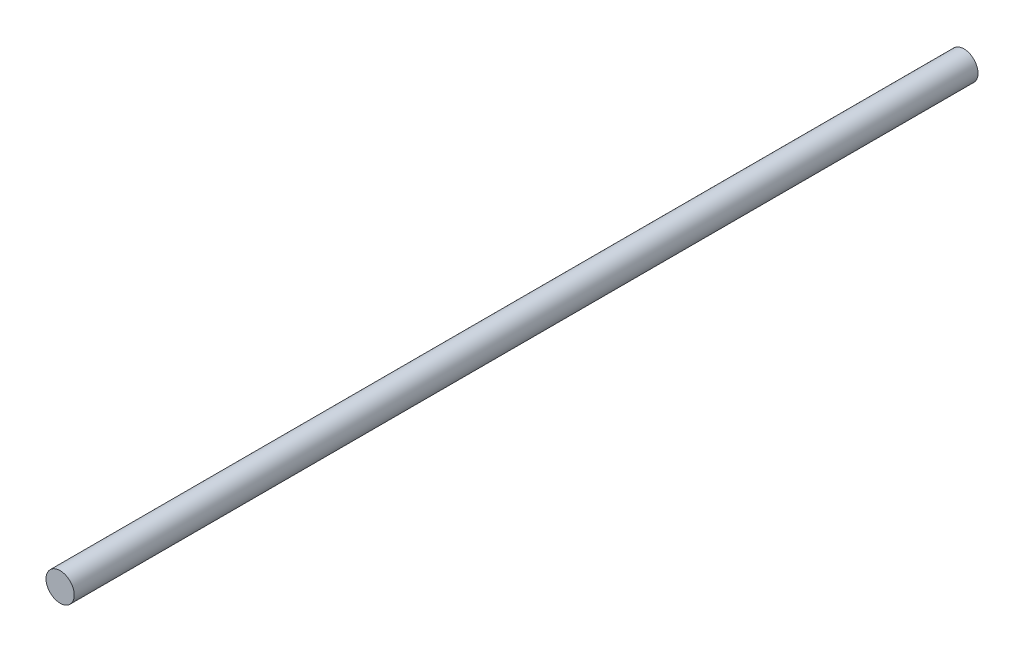
SolidWorks part; units mm, degrees
ref_plane "Front Plane" through (0, 0, 0) normal (0, 0, 1) x (1, 0, 0)
ref_plane "Top Plane" through (0, 0, 0) normal (0, 1, 0) x (1, 0, 0)
ref_plane "Right Plane" through (0, 0, 0) normal (1, 0, 0) x (0, 0, -1)
other "Configuration Table"
sketch "Sketch1" plane through (0, 0, 0) normal (0, 0, 1) x (1, 0, 0)
  circle A0 centre (0, 0) radius 5
  dimension "D1" = 10
extrude "Boss-Extrude1" add sketch "Sketch1" along normal blind 320
sketch "Sketch3" plane through (0, 0, 0) normal (0, 1, 0) x (1, 0, 0)
  line L0 (0, 0) -> (0, -320)
  line L1 (-5, -320) -> (5, -320) construction
